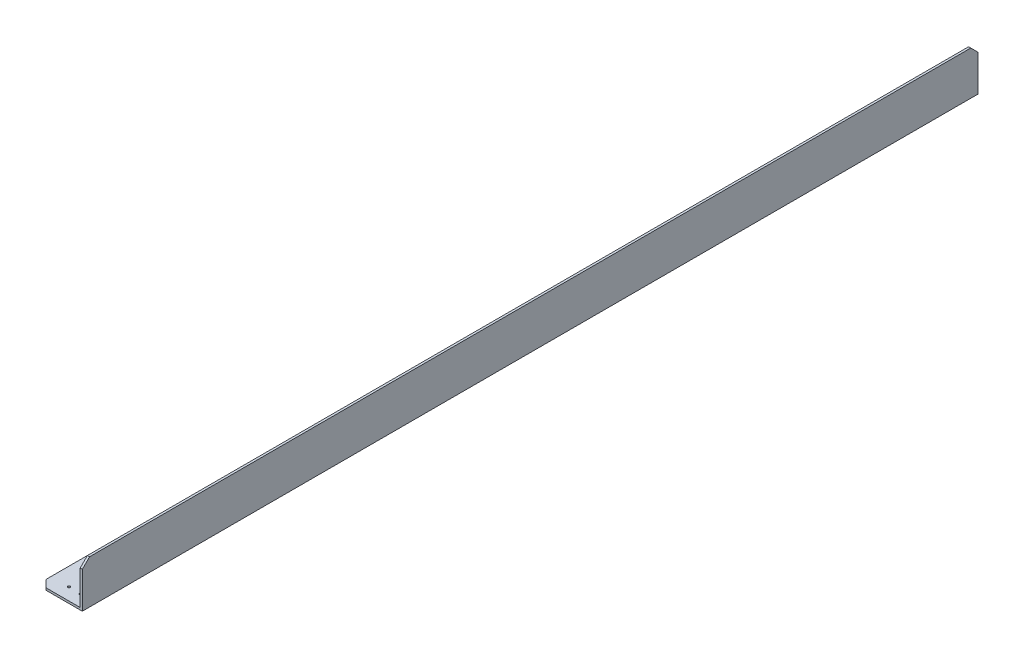
from build123d import *

# Parameters (mm, degrees)
EXTRUDE_1_DEPTH        = 617
HOLE_WIZARD_M4_2_D     = 3.3
HOLE_WIZARD_M4_3_D     = 3.3
HOLE_WIZARD_M4_3_DEPTH = 3
HOLE_WIZARD_M4_1_D     = 4.8
HOLE_WIZARD_M4_4_D     = 3.3
CHAMFER_1_SIZE         = 10


with BuildPart() as part:
    # 草图1 → 凸台-拉伸1 (new, symmetric)
    with BuildSketch(Plane.XY):
        Polygon((0, 0), (60, 0), (60, 60), (57, 60), (57, 3), (0, 3), align=None)
    extrude(amount=EXTRUDE_1_DEPTH, both=True)

    # M4 螺纹孔2 (through all)
    with Locations(Plane(origin=(0, 3, 0), x_dir=(1, 0, 0), z_dir=(0, 1, 0))):
        with Locations((24.75, 499.931449769), (9.75, 484.931449769), (39.75, 484.931449769), (39.75, -484.931449769), (9.75, -484.931449769), (24.75, -499.931449769)):
            Hole(HOLE_WIZARD_M4_2_D / 2)

    # M4 螺纹孔3
    with Locations(Plane(origin=(0, 3, 0), x_dir=(1, 0, 0), z_dir=(0, 1, 0))):
        with Locations((9.75, 484.931449769), (39.75, 484.931449769), (24.75, 469.931449769), (24.75, 499.931449769), (24.75, -499.931449769), (24.75, -469.931449769), (39.75, -484.931449769), (9.75, -484.931449769)):
            Hole(HOLE_WIZARD_M4_3_D / 2, depth=HOLE_WIZARD_M4_3_DEPTH)

    # M4 间隙孔1 (through all)
    with Locations(Plane(origin=(0, 3, 0), x_dir=(1, 0, 0), z_dir=(0, 1, 0))):
        with Locations((42, 0), (42, 200), (42, 400), (42, 600), (42, -600), (42, -400), (42, -200)):
            Hole(HOLE_WIZARD_M4_1_D / 2)

    # M4 螺纹孔4 (through all)
    with Locations(Plane(origin=(0, 3, 0), x_dir=(1, 0, 0), z_dir=(0, 1, 0))):
        with Locations((24.75, 0), (24.75, 120), (24.75, 240), (24.75, 360), (24.75, 480), (24.75, 600), (24.75, -600), (24.75, -480), (24.75, -360), (24.75, -240), (24.75, -120)):
            Hole(HOLE_WIZARD_M4_4_D / 2)

    # 倒角1
    chamfer_1_edges = [part.edges().sort_by_distance(p)[0] for p in [
        (58.5, 60, 617),
        (0, 1.5, 617),
        (58.5, 60, -617),
        (0, 1.5, -617),
    ]]
    chamfer(chamfer_1_edges, length=CHAMFER_1_SIZE)


solid = part.part
